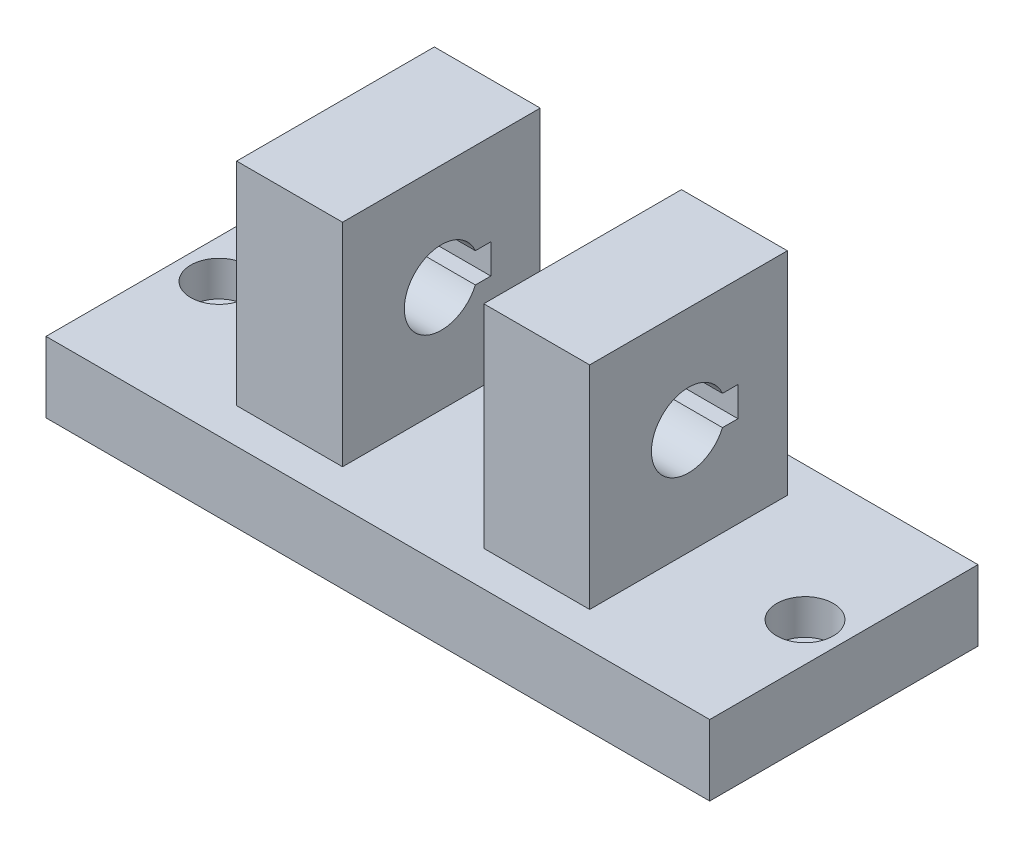
from build123d import *

# Parameters (mm, degrees)
SKETCH1_W           = 94
SKETCH1_H           = 38
BOSS_EXTRUDE1_DEPTH = 10
SKETCH2_R           = 4
CUT_EXTRUDE1_DEPTH  = 5
SKETCH3_R           = 2.5
CUT_EXTRUDE2_DEPTH  = 5
SKETCH4_W           = 28
SKETCH4_H           = 30
BOSS_EXTRUDE2_DEPTH = 15
CUT_EXTRUDE3_DEPTH  = 109
CUT_EXTRUDE4_DEPTH  = 70


with BuildPart() as part:
    # Sketch1 → Boss-Extrude1 (new body)
    with BuildSketch(Plane(origin=(0, 0, 0), x_dir=(1, 0, 0), z_dir=(0, 1, 0))):
        Rectangle(SKETCH1_W, SKETCH1_H)
    extrude(amount=BOSS_EXTRUDE1_DEPTH)

    # Sketch2 → Cut-Extrude1 (cut)
    with BuildSketch(Plane(origin=(0, 10, 0), x_dir=(1, 0, 0), z_dir=(0, 1, 0))):
        with Locations(Location((-41.5, 0, 0), (0, 0, 270))):
            Circle(SKETCH2_R)
    cut_extrude1 = extrude(amount=-CUT_EXTRUDE1_DEPTH, mode=Mode.SUBTRACT)

    # Sketch3 → Cut-Extrude2 (cut)
    with BuildSketch(Plane(origin=(0, 5, 0), x_dir=(1, 0, 0), z_dir=(0, 1, 0))):
        with Locations(Location((-41.5, 0, 0), (0, 0, 270))):
            Circle(SKETCH3_R)
    cut_extrude2 = extrude(amount=-CUT_EXTRUDE2_DEPTH, mode=Mode.SUBTRACT)

    # Sketch4 → Boss-Extrude2 (add)
    with BuildSketch(Plane.ZY.offset(25)):
        with Locations((0, 25)):
            Rectangle(SKETCH4_W, SKETCH4_H)
    boss_extrude2 = extrude(amount=-BOSS_EXTRUDE2_DEPTH)

    # Sketch6 → Cut-Extrude3 (cut)
    with BuildSketch(Plane.ZY.offset(25)):
        with BuildLine():
            Line((-7, 27.1), (-4.81170448, 27.1))
            ThreePointArc((-4.81170448, 27.1), (5.25, 25), (-4.81170448, 22.9))
            Line((-4.81170448, 22.9), (-7, 22.9))
            Line((-7, 22.9), (-7, 27.1))
        make_face()
    extrude(amount=-CUT_EXTRUDE3_DEPTH, mode=Mode.SUBTRACT)

    # Mirror1: Cut-Extrude1, Cut-Extrude2, Boss-Extrude2 across plane
    add(cut_extrude1.mirror(Plane(origin=(0, 0, 0), x_dir=(0, 0, 1), z_dir=(1, 0, 0))), mode=Mode.SUBTRACT)
    add(cut_extrude2.mirror(Plane(origin=(0, 0, 0), x_dir=(0, 0, 1), z_dir=(1, 0, 0))), mode=Mode.SUBTRACT)
    add(boss_extrude2.mirror(Plane(origin=(0, 0, 0), x_dir=(0, 0, 1), z_dir=(1, 0, 0))))

    # Sketch7 → Cut-Extrude4 (cut)
    with BuildSketch(Plane.ZY.offset(-10)):
        with BuildLine():
            Line((-7, 22.9), (-4.81170448, 22.9))
            ThreePointArc((-4.81170448, 22.9), (5.25, 25), (-4.81170448, 27.1))
            Line((-4.81170448, 27.1), (-7, 27.1))
            Line((-7, 27.1), (-7, 22.9))
        make_face()
    extrude(amount=-CUT_EXTRUDE4_DEPTH, mode=Mode.SUBTRACT)


solid = part.part
